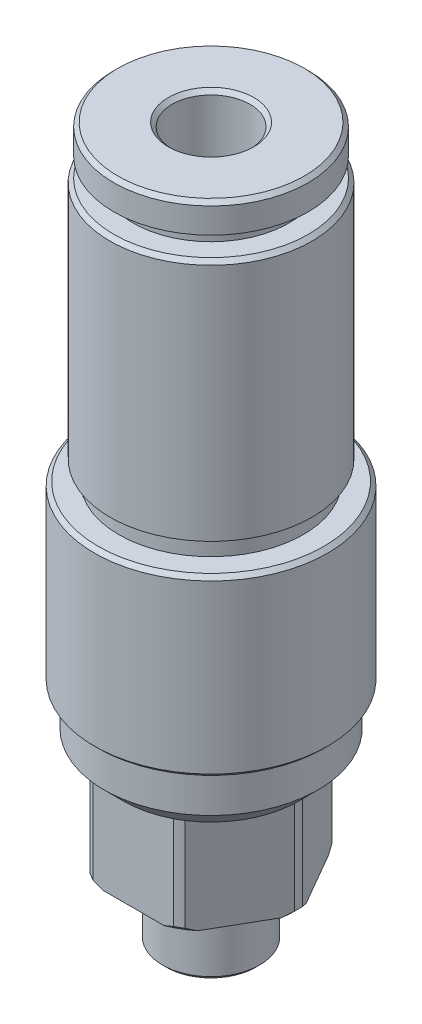
SolidWorks part; units mm, degrees
material "聚氨脂"
ref_plane "Front Plane" through (0, 0, 0) normal (0, 0, 1) x (1, 0, 0)
ref_plane "Top Plane" through (0, 0, 0) normal (0, 1, 0) x (1, 0, 0)
ref_plane "Right Plane" through (0, 0, 0) normal (1, 0, 0) x (0, 0, -1)
sketch "Sketch1" plane through (0, 0, 0) normal (0, 0, 1) x (1, 0, 0)
  line L0 (1.45, 0) -> (2.3, 0)
  line L1 (2.5, 0.2) -> (2.5, 3)
  line L2 (2.5, 3) -> (2, 3)
  line L3 (2, 3) -> (2, 3.5)
  line L4 (2, 3.5) -> (4.3, 3.5)
  line L5 (4.5, 3.7) -> (4.5, 8.5)
  line L6 (4.5, 8.5) -> (5.5, 9.5)
  line L7 (5.5, 9.5) -> (5.5, 11.5)
  line L8 (5.5, 11.5) -> (5.8, 11.5)
  line L9 (6, 11.7) -> (6, 20.3)
  line L10 (5.8, 20.5) -> (4.75, 20.5)
  line L11 (4.75, 20.5) -> (4.75, 21.5)
  line L12 (4.75, 21.5) -> (5.2, 21.5)
  line L13 (5.2, 21.5) -> (5.2, 33.8)
  line L14 (5, 34) -> (4, 34)
  line L15 (4, 34) -> (4, 35)
  line L16 (4, 35) -> (5, 35)
  line L17 (5, 35) -> (5, 36.3)
  line L18 (4.8, 36.5) -> (2.2, 36.5)
  line L19 (1.25, 5) -> (1.25, 0.2)
  line L20 (0, 0) -> (0, 7.2924) construction
  line L21 (1.25, 0.2) -> (1.45, 0)
  line L24 (1.25, 5) -> (2, 5.75)
  line L25 (2, 36.3) -> (2, 5.75)
  line L26 (2.3, 0) -> (2.5, 0.2)
  line L27 (4.3, 3.5) -> (4.5, 3.7)
  line L28 (2.2, 36.5) -> (2, 36.3)
  line L29 (5, 36.3) -> (4.8, 36.5)
  line L30 (5.2, 33.8) -> (5, 34)
  line L31 (6, 20.3) -> (5.8, 20.5)
  line L32 (5.8, 11.5) -> (6, 11.7)
  point P0 (1.25, 0)
  point P1 (2.5, 0)
  point P7 (4.5, 3.5)
  point P11 (6, 11.5)
  point P12 (6, 20.5)
  point P16 (5.2, 34)
  point P20 (5, 36.5)
  point P34 (2, 36.5)
  dimension "D1" = 2.5
  dimension "D2" = 5
  dimension "D3" = 10.4
  dimension "D4" = 12
  dimension "D5" = 10
  dimension "D6" = 8
  dimension "D7" = 9.5
  dimension "D8" = 11
  dimension "D9" = 9
  dimension "D10" = 0.5
  dimension "D11" = 0.5
  dimension "D12" = 16
  dimension "D13" = 1.5
  dimension "D14" = 1
  dimension "D15" = 36.5
  dimension "D16" = 1
  dimension "D17" = 33
  dimension "D18" = 1
  dimension "D19" = 2
  dimension "D20" = 9
  dimension "D21" = 4
  dimension "D22" = 0.75
  dimension "D23" = 5
  dimension "D24" = 5
revolve "Revolve1" add sketch "Sketch1" angle 360 about L20
cosmetic thread "Cosmetic Thread1" parameters "D1"=3, "D2"=4.134
sketch "Sketch3" plane through (0, 3.5, 0) normal (0, -1, 0) x (1, 0, 0)
  line L1 (2.3094, -4) -> (4.6188, 0)
  line L2 (4.6188, 0) -> (2.3094, 4)
  line L3 (2.3094, 4) -> (-2.3094, 4)
  line L4 (-2.3094, 4) -> (-4.6188, 0)
  line L5 (-4.6188, 0) -> (-2.3094, -4)
  line L6 (-2.3094, -4) -> (2.3094, -4)
  circle A0 centre (0, 0) radius 4 construction
  dimension "D1" = 8
extrude "Cut-Extrude1" cut sketch "Sketch3" against normal blind 5 flip side to cut
